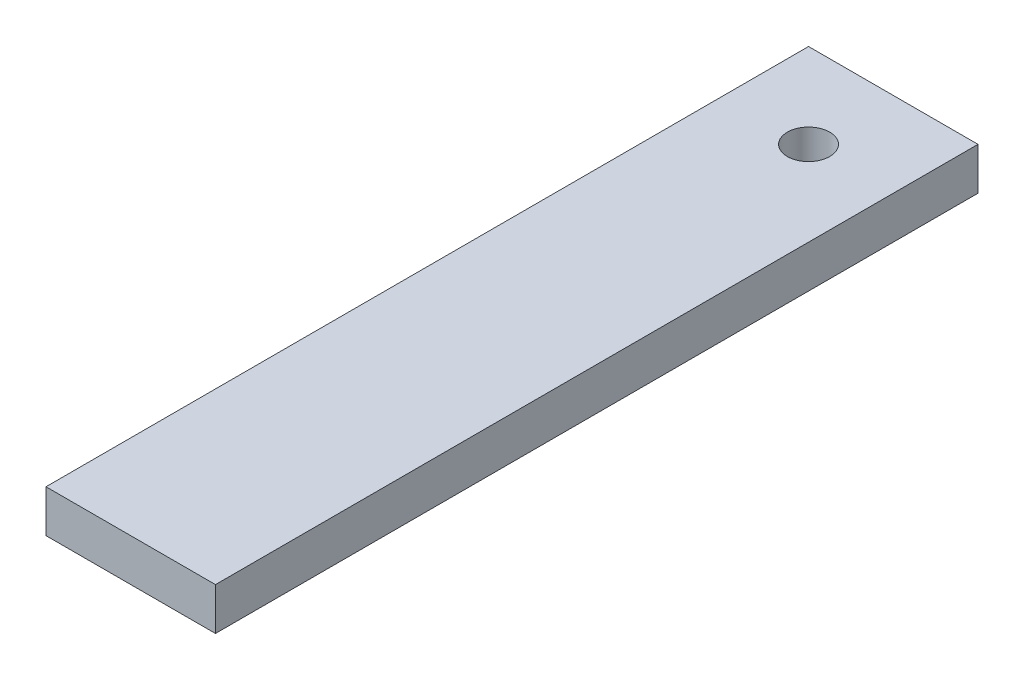
from build123d import *

# Parameters (mm, degrees)
SKETCH1_W           = 20
SKETCH1_H           = 90
SKETCH1_R           = 2.5
BOSS_EXTRUDE1_DEPTH = 5


with BuildPart() as part:
    # Sketch1 → Boss-Extrude1 (new body)
    with BuildSketch(Plane(origin=(0, 0, 0), x_dir=(1, 0, 0), z_dir=(0, 1, 0))):
        Rectangle(SKETCH1_W, SKETCH1_H)
        with Locations(Location((0, 35, 0), (0, 0, 270))):
            Circle(SKETCH1_R, mode=Mode.SUBTRACT)
    extrude(amount=BOSS_EXTRUDE1_DEPTH)


solid = part.part
